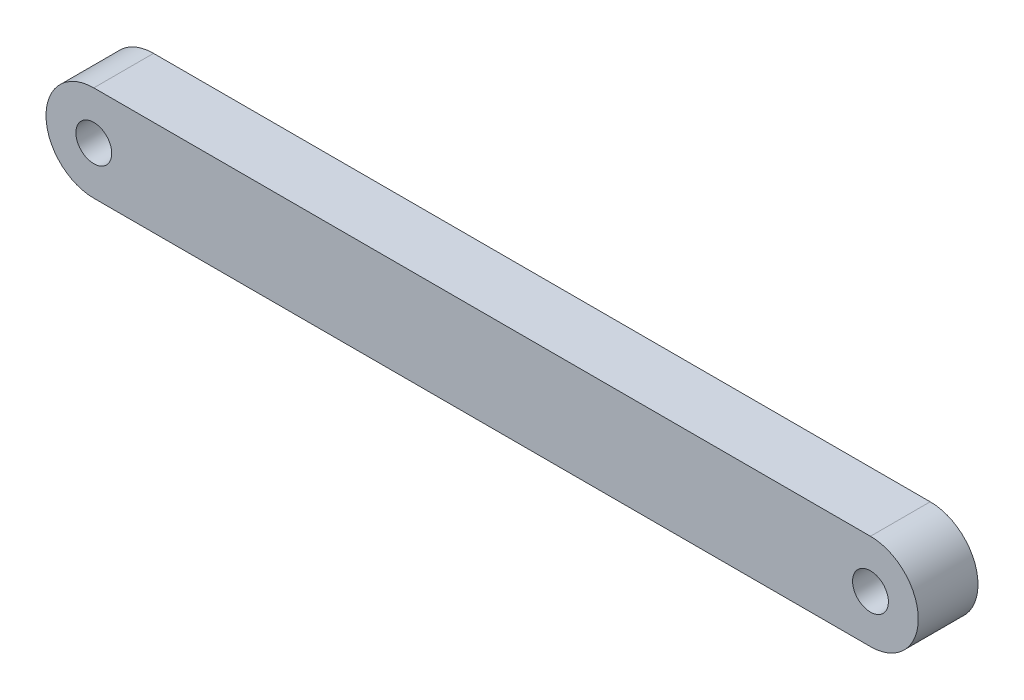
SolidWorks part; units mm, degrees
material "1.0503 (C45)"
ref_plane "Front Plane" through (0, 0, 0) normal (0, 0, 1) x (1, 0, 0)
ref_plane "Top Plane" through (0, 0, 0) normal (0, 1, 0) x (1, 0, 0)
ref_plane "Right Plane" through (0, 0, 0) normal (1, 0, 0) x (0, 0, -1)
sketch "Sketch1" plane through (0, 0, 0) normal (0, 0, 1) x (1, 0, 0)
  line L0 (-32.5, 0) -> (32.5, 0) construction
  line L1 (-32.5, 4) -> (32.5, 4)
  line L2 (-32.5, -4) -> (32.5, -4)
  arc A0 (-32.5, 4) -> (-32.5, -4) centre (-32.5, 0) ccw
  arc A1 (32.5, -4) -> (32.5, 4) centre (32.5, 0) ccw
  point P2 (0, 0)
  dimension "D2" = 4
  dimension "D1" = 65
extrude "Boss-Extrude1" add sketch "Sketch1" along normal blind 5
sketch "Sketch3" plane through (0, 0, 5) normal (0, 0, 1) x (1, 0, 0)
  circle A0 centre (-32.5, 0) radius 1.5
  circle A1 centre (32.5, 0) radius 1.5
  arc A2 (-32.5, 4) -> (-32.5, -4) centre (-32.5, 0) ccw construction
  arc A3 (32.5, -4) -> (32.5, 4) centre (32.5, 0) ccw construction
  dimension "D1" = 3
extrude "Cut-Extrude1" cut sketch "Sketch3" against normal through all
